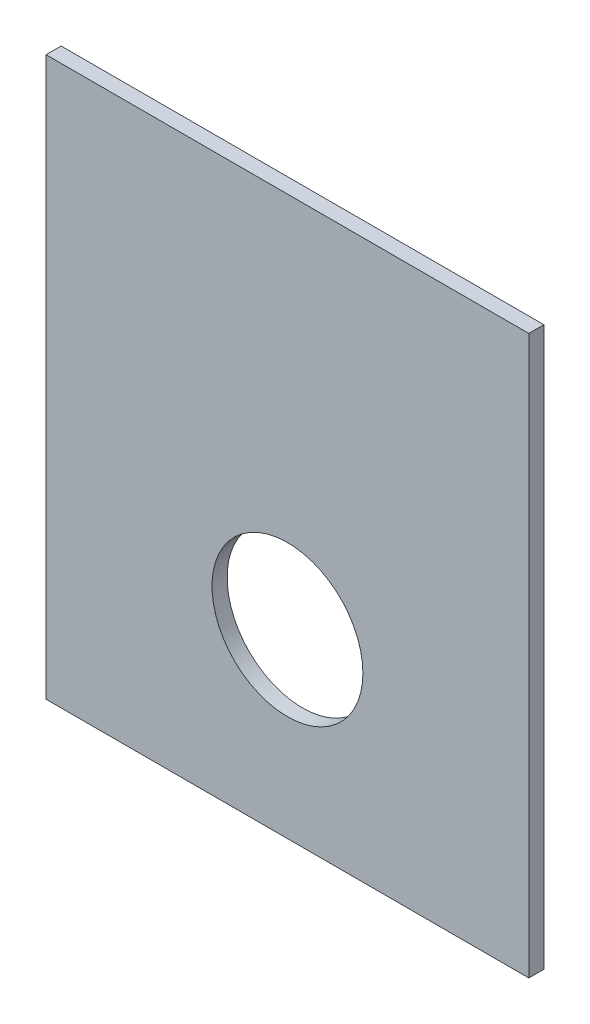
from build123d import *

# Parameters (mm, degrees)
SKETCH1_W           = 320
SKETCH1_H           = 370
SKETCH1_R           = 50
BOSS_EXTRUDE1_DEPTH = 10


with BuildPart() as part:
    # Sketch1 → Boss-Extrude1 (new body)
    with BuildSketch(Plane.XY):
        with Locations((160, 185)):
            Rectangle(SKETCH1_W, SKETCH1_H)
        with Locations((160, 120)):
            Circle(SKETCH1_R, mode=Mode.SUBTRACT)
    extrude(amount=BOSS_EXTRUDE1_DEPTH)


solid = part.part
